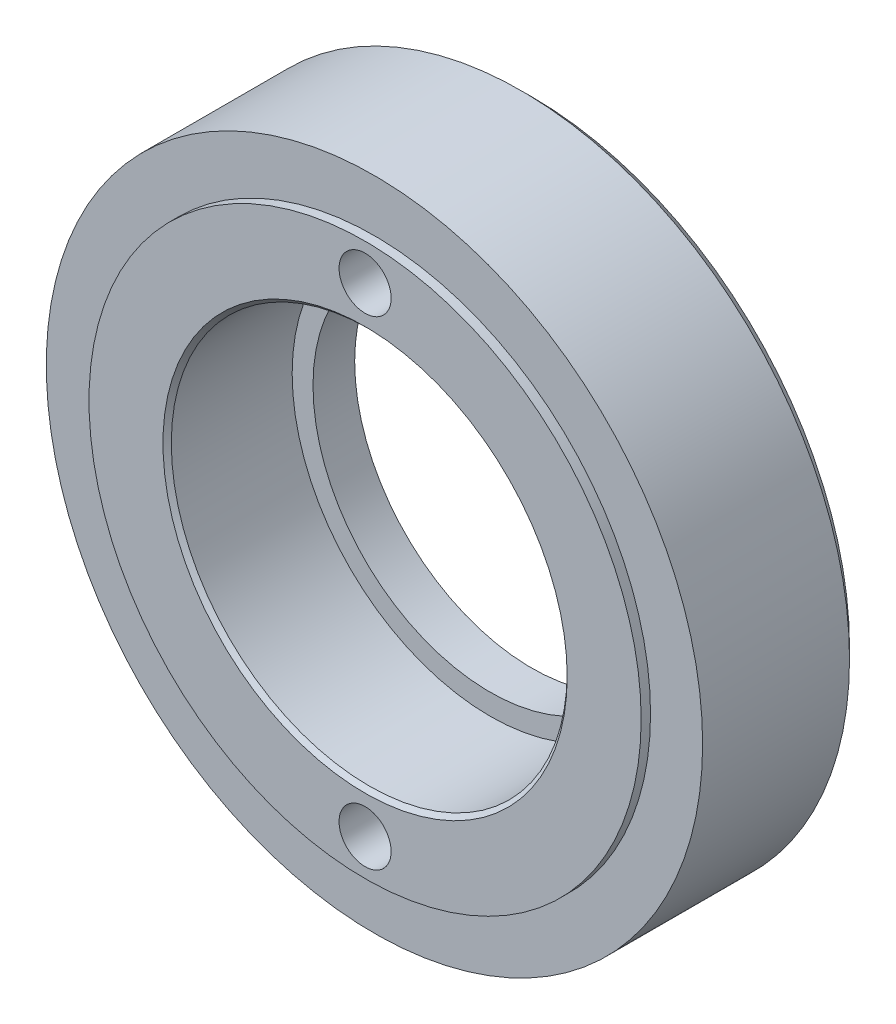
SolidWorks part; units mm, degrees
ref_plane "Front Plane" through (0, 0, 0) normal (0, 0, 1) x (1, 0, 0)
ref_plane "Top Plane" through (0, 0, 0) normal (0, 1, 0) x (1, 0, 0)
ref_plane "Right Plane" through (0, 0, 0) normal (1, 0, 0) x (0, 0, -1)
sketch "Sketch1" plane through (0, 0, 0) normal (0, 0, 1) x (1, 0, 0)
  circle A0 centre (0, 0) radius 15.75
  circle A1 centre (0, 0) radius 9.5
  dimension "D1" = 31.5
  dimension "D2" = 19
extrude "Boss-Extrude1" add sketch "Sketch1" along normal mid plane 8
sketch "Sketch2" plane through (0, 0, 0) normal (0, 0, 1) x (1, 0, 0)
  circle A0 centre (0, 0) radius 10
  circle A1 centre (0, 0) radius 9.5
  dimension "D1" = 20
sketch "Sketch3" plane through (0, 0, -4) normal (0, 0, -1) x (-1, 0, 0)
  circle A0 centre (0, 0) radius 8.5
  circle A1 centre (0, 0) radius 10.6391
  dimension "D1" = 17
extrude "Boss-Extrude2" add sketch "Sketch3" against normal blind 2
hole_wizard "M3 Tapped Hole1" positions "Sketch4" profile "Sketch5" tap size "M3" standard "GB" end condition through all
sketch "Sketch4" plane through (0, 0, 4) normal (0, 0, 1) x (1, 0, 0)
  point P0 (0, -11.5)
  dimension "D1" = 11.5
sketch "Sketch5" plane through (0, -11.5, 4) normal (1, 0, 0) x (0, -1, 0)
  line L0 (0, 0) -> (0, 8)
  line L1 (0, 8) -> (1.25, 8)
  line L2 (1.25, 8) -> (1.25, 0)
  line L5 (1.25, 0) -> (0, 0)
  line L11 (0, -6.35) -> (0, 107.95) construction
  dimension "通孔螺纹孔钻头直径" = 2.5
  dimension "通孔螺纹孔钻头深度" = 8
cosmetic thread "Hole thread1" parameters "D2"=3
mirror "Mirror1" about plane through (0, 0, 0) normal (0, 1, 0) of "M3 Tapped Hole1"
chamfer "Chamfer1" distance 0.2 angle 45 1 edges at (9.5, 0, 4)
sketch "Sketch6" plane through (0, 0, 4) normal (0, 0, 1) x (1, 0, 0)
  circle A0 centre (0, 0) radius 13.25
  circle A1 centre (0, 0) radius 20.677
  dimension "D1" = 26.5
extrude "Cut-Extrude1" cut sketch "Sketch6" against normal blind 0.45
chamfer "Chamfer2" distance 0.5 angle 45 1 edges at (15.75, 0, -4)
